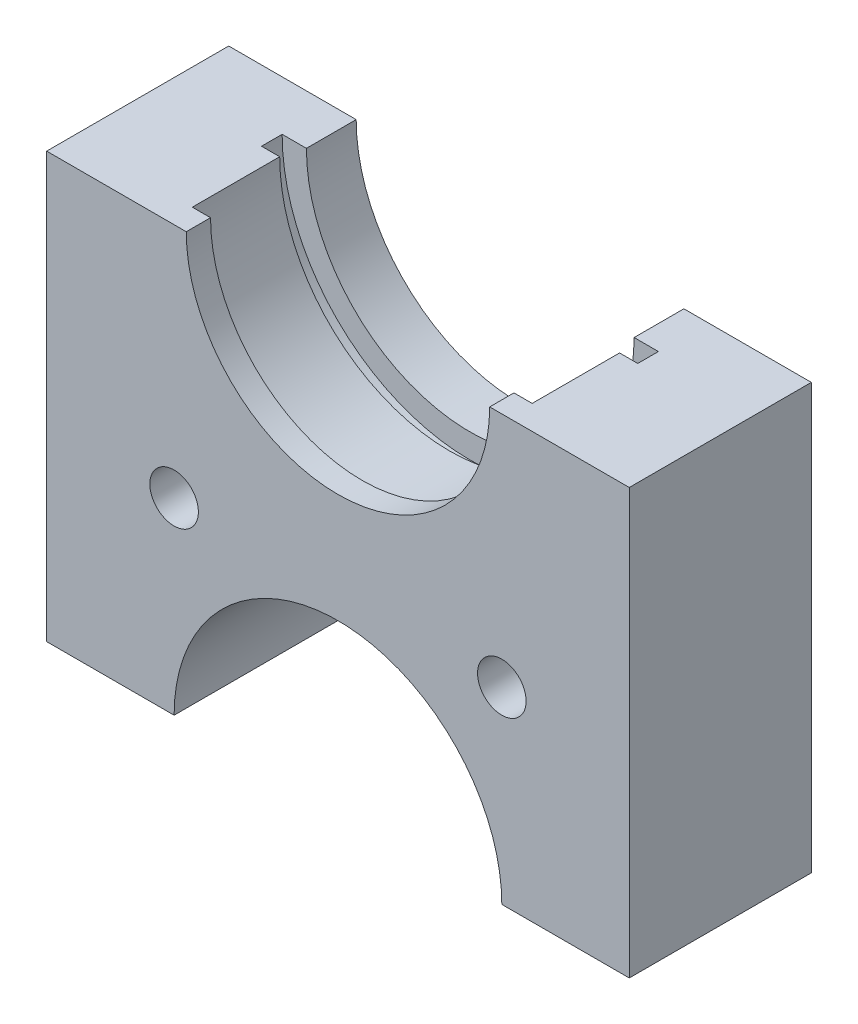
from build123d import *

# Parameters (mm, degrees)
SKETCH_1_W               = 480
SKETCH_1_H               = 350
EXTRUDE_1_DEPTH          = 150
CUT_EXTRUDE_1_DEPTH      = 333.753662639
CUT_EXTRUDE_1_DEPTH_BACK = 333.753662639
SKETCH_2_R               = 20
CUT_EXTRUDE_2_DEPTH      = 333.753662639
CUT_EXTRUDE_2_DEPTH_BACK = 333.753662639
SKETCH_3_R               = 135
SKETCH_3_R_2             = 125


with BuildPart() as part:
    # 草图1 → 凸台-拉伸1 (new body)
    with BuildSketch(Plane.XY):
        Rectangle(SKETCH_1_W, SKETCH_1_H)
    extrude(amount=EXTRUDE_1_DEPTH)

    # 草图2 → 切除-拉伸1 (cut, two sides: drawn at the far end of the back side and taken through both)
    with BuildSketch(Plane.XY.offset(150).offset(-CUT_EXTRUDE_1_DEPTH_BACK)):
        with Locations((-135, -20)):
            Circle(SKETCH_2_R)
        with Locations((135, -20)):
            Circle(SKETCH_2_R)
    extrude(amount=CUT_EXTRUDE_1_DEPTH + CUT_EXTRUDE_1_DEPTH_BACK, mode=Mode.SUBTRACT)

    # 草图3 → 切除-拉伸2 (cut, two sides: drawn at the far end of the back side and taken through both)
    with BuildSketch(Plane.XY.offset(150).offset(-CUT_EXTRUDE_2_DEPTH_BACK)):
        with Locations((0, -175)):
            Circle(SKETCH_3_R)
        with Locations((0, 175)):
            Circle(SKETCH_3_R_2)
    extrude(amount=CUT_EXTRUDE_2_DEPTH + CUT_EXTRUDE_2_DEPTH_BACK, mode=Mode.SUBTRACT)

    # 草图5 → 切除-旋转1 (revolve, cut)
    with BuildSketch(Plane(origin=(0, 175, 0), x_dir=(1, 0, 0), z_dir=(0, 1, 0))):
        Polygon((0, -130), (-140, -130), (-140, -58), (-155, -58), (-155, -41), (-135, -41), (-135, 0), (0, 0), (0, -41), align=None)
    revolve(axis=Axis((0, 175, 150), (0, 0, -1)), mode=Mode.SUBTRACT)


solid = part.part
